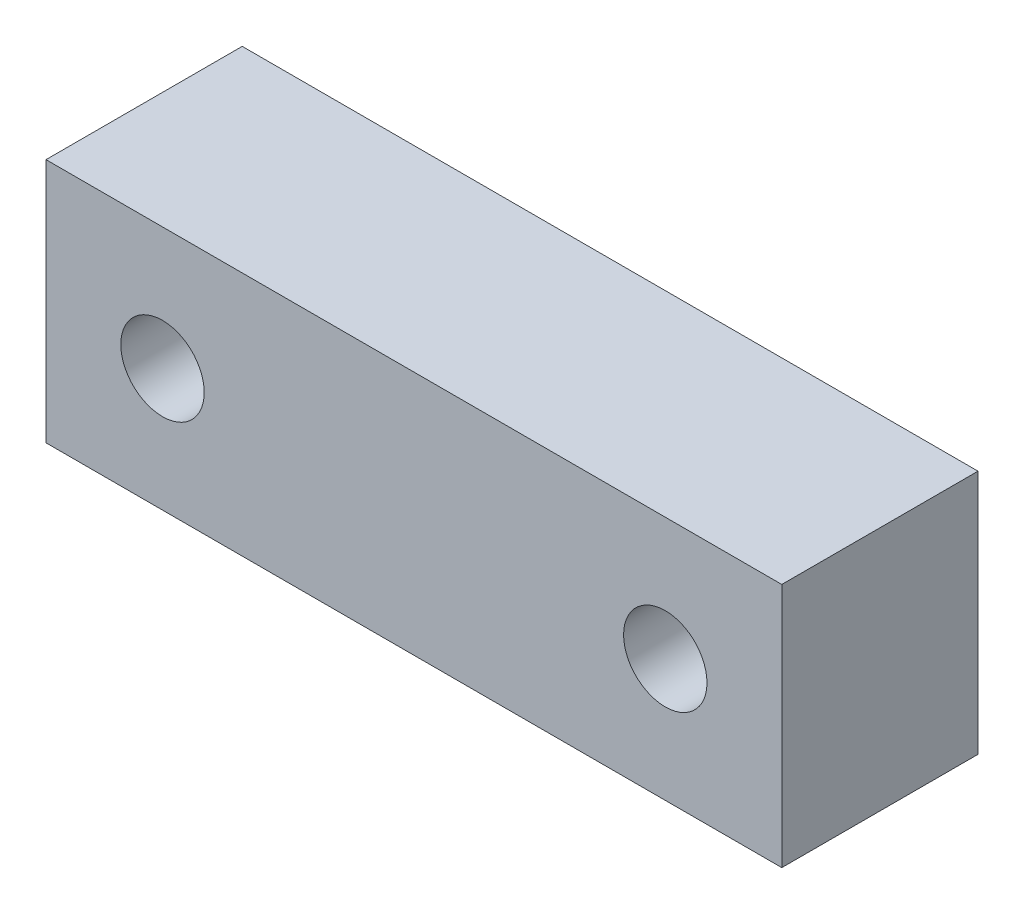
SolidWorks part; units mm, degrees
ref_plane "前视基准面" through (0, 0, 0) normal (0, 0, 1) x (1, 0, 0)
ref_plane "上视基准面" through (0, 0, 0) normal (0, 1, 0) x (1, 0, 0)
ref_plane "右视基准面" through (0, 0, 0) normal (1, 0, 0) x (0, 0, -1)
sketch "草图1" plane through (0, 0, 0) normal (0, 0, 1) x (1, 0, 0)
  line L1 (15, -5) -> (-15, -5)
  line L2 (15, -5) -> (15, 5)
  line L3 (15, 5) -> (-15, 5)
  line L4 (-15, -5) -> (-15, 5)
  line L5 (15, -5) -> (-15, 5) construction
  line L6 (15, 5) -> (-15, -5) construction
  point P0 (0, 0)
  dimension "D1" = 30
  dimension "D2" = 10
extrude "凸台-拉伸1" add sketch "草图1" along normal blind 8
hole_wizard "打孔尺寸(%根据)内六角圆柱头螺钉的类型1" positions "草图2" profile "草图3" counterbore size "M3" standard "GB" end condition up to next
sketch "草图2" plane through (0, 0, 0) normal (0, 0, -1) x (-1, 0, 0)
  point P0 (-10.25, 0)
  point P3 (10.25, 0)
sketch "草图3" plane through (10.25, 0, 0) normal (1, 0, 0) x (0, 1, 0)
  line L0 (0, 0) -> (0, 8)
  line L1 (0, 8) -> (1.7, 8)
  line L3 (1.7, 8) -> (1.7, 3.4)
  line L4 (1.7, 3.4) -> (3, 3.4)
  line L5 (3, 3.4) -> (3, 0)
  line L7 (3, 0) -> (0, 0)
  line L11 (0, -6.35) -> (0, 107.95) construction
  dimension "通孔孔直径" = 3.4
  dimension "通孔孔深度" = 8
  dimension "柱形沉头孔直径" = 6
  dimension "柱形沉头孔深度" = 3.4
